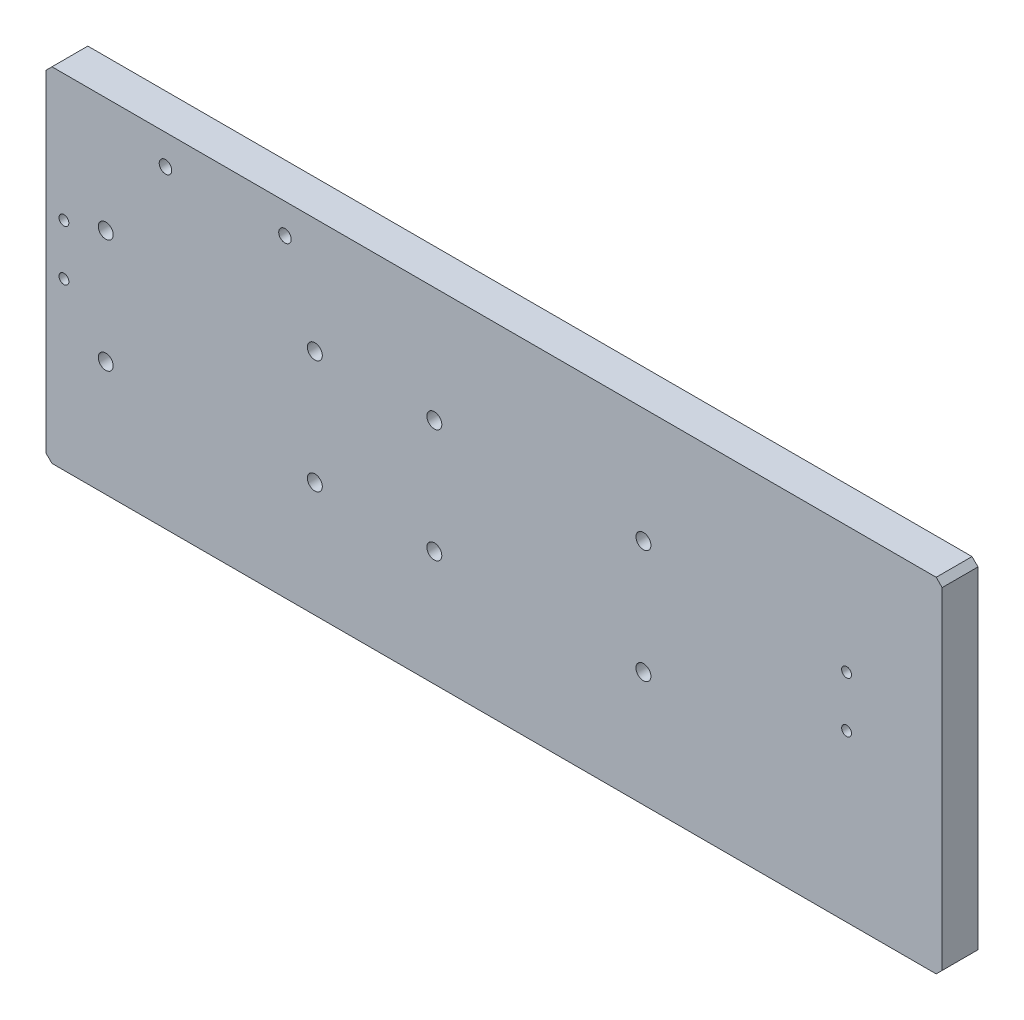
SolidWorks part; units mm, degrees
material "A6061"
ref_plane "前基準面" through (0, 0, 0) normal (0, 0, 1) x (1, 0, 0)
ref_plane "上基準面" through (0, 0, 0) normal (0, 1, 0) x (1, 0, 0)
ref_plane "右基準面" through (0, 0, 0) normal (1, 0, 0) x (0, 0, -1)
sketch "草图1" plane through (0, 0, 0) normal (0, 0, 1) x (1, 0, 0)
  line L1 (-150, -57.5) -> (150, -57.5)
  line L2 (-150, -57.5) -> (-150, 57.5)
  line L3 (-150, 57.5) -> (150, 57.5)
  line L4 (150, -57.5) -> (150, 57.5)
  line L5 (-150, -57.5) -> (150, 57.5) construction
  line L6 (-150, 57.5) -> (150, -57.5) construction
  point P0 (0, 0)
  dimension "D1" = 115
  dimension "D2" = 300
extrude "凸台-拉伸1" add sketch "草图1" along normal blind 12
sketch "草图4" plane through (0, 0, 0) normal (0, 0, -1) x (-1, 0, 0)
  line L0 (0, 0) -> (168.5016, 0) construction
  line L2 (150, 57.5) -> (150, -57.5) construction
  line L3 (-150, -57.5) -> (-150, 57.5) construction
  point P0 (130, 19)
  point P3 (60, -19)
  point P12 (60, 19)
  point P14 (130, -19)
  point P19 (20, 19)
  point P20 (-50, -19)
  point P21 (-50, 19)
  point P22 (20, -19)
  dimension "D1" = 2
  dimension "D2" = 38
  dimension "D3" = 70
  dimension "D4" = 20
  dimension "D5" = 100
hole_wizard "M6 螺纹孔1" positions "草图4" profile "草图5" tap size "M6" standard "GB" end condition through all
sketch "草图5" plane through (-130, 19, 0) normal (1, 0, 0) x (0, 1, 0)
  line L0 (0, 0) -> (0, 12)
  line L1 (0, 12) -> (2.5, 12)
  line L2 (2.5, 12) -> (2.5, 0)
  line L5 (2.5, 0) -> (0, 0)
  line L11 (0, -6.35) -> (0, 107.95) construction
  dimension "通孔螺纹孔钻头直径" = 5
  dimension "通孔螺纹孔钻头深度" = 12
cosmetic thread "孔螺纹线17" parameters "D2"=6
cosmetic thread "孔螺纹线18" parameters "D2"=6
cosmetic thread "孔螺纹线19" parameters "D2"=6
cosmetic thread "孔螺纹线20" parameters "D2"=6
cosmetic thread "孔螺纹线21" parameters "D2"=6
cosmetic thread "孔螺纹线22" parameters "D2"=6
cosmetic thread "孔螺纹线23" parameters "D2"=6
cosmetic thread "孔螺纹线24" parameters "D2"=6
sketch "草图6" plane through (0, 0, 12) normal (0, 0, 1) x (1, 0, 0)
  line L0 (-150, 57.5) -> (-150, -57.5) construction
  line L2 (150, 57.5) -> (-150, 57.5) construction
  line L3 (150, -57.5) -> (150, 57.5) construction
  point P0 (-144, 15)
  point P3 (-144, -2)
  point P6 (118, 15)
  point P9 (118, -2)
  dimension "D1" = 6
  dimension "D2" = 262
  dimension "D3" = 42.5
  dimension "D4" = 17
  dimension "D5" = 32
hole_wizard "M4 螺纹孔2" positions "草图6" profile "草图7" tap size "M4" standard "GB" end condition through all
sketch "草图7" plane through (-144, 15, 12) normal (1, 0, 0) x (0, -1, 0)
  line L0 (0, 0) -> (0, 12)
  line L1 (0, 12) -> (1.65, 12)
  line L2 (1.65, 12) -> (1.65, 0)
  line L5 (1.65, 0) -> (0, 0)
  line L11 (0, -6.35) -> (0, 107.95) construction
  dimension "通孔螺纹孔钻头直径" = 3.3
  dimension "通孔螺纹孔钻头深度" = 12
cosmetic thread "孔螺纹线28" parameters "D2"=4
cosmetic thread "孔螺纹线29" parameters "D2"=4
cosmetic thread "孔螺蚊线1" parameters "D2"=4
cosmetic thread "孔螺蚊线2" parameters "D2"=4
sketch "草图10" plane through (0, 0, 0) normal (0, 0, -1) x (-1, 0, 0)
  line L1 (-150, 57.5) -> (150, 57.5) construction
  line L2 (-150, -57.5) -> (-150, 57.5) construction
  point P0 (110, 47.5)
  point P2 (70, 47.5)
  dimension "D1" = 40
  dimension "D2" = 220
  dimension "D3" = 10
hole_wizard "M5 螺纹孔1" positions "草图10" profile "草图11" tap size "M5" standard "GB" end condition through all
sketch "草图11" plane through (-110, 47.5, 0) normal (1, 0, 0) x (0, 1, 0)
  line L0 (0, 0) -> (0, 12)
  line L1 (0, 12) -> (2.1, 12)
  line L2 (2.1, 12) -> (2.1, 0)
  line L5 (2.1, 0) -> (0, 0)
  line L11 (0, -6.35) -> (0, 107.95) construction
  dimension "通孔螺纹孔钻头直径" = 4.2
  dimension "通孔螺纹孔钻头深度" = 12
cosmetic thread "孔螺纹线35" parameters "D2"=5
cosmetic thread "孔螺纹线36" parameters "D2"=5
chamfer "倒角1" distance 2 angle 45 4 edges at (150, 57.5, 6) (150, -57.5, 6) (-150, 57.5, 6) (-150, -57.5, 6)
